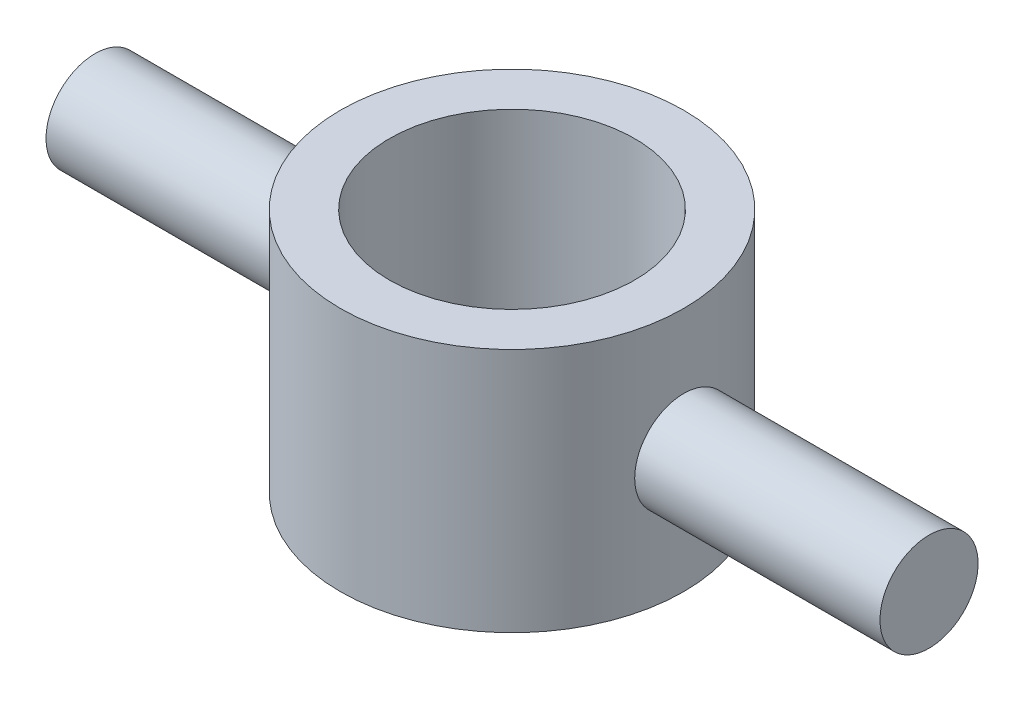
from build123d import *

# Parameters (mm, degrees)
SKETCH_2_R      = 7
SKETCH_2_R_2    = 5
EXTRUDE_1_DEPTH = 10
SKETCH_3_R      = 2
EXTRUDE_2_DEPTH = 10


with BuildPart() as part:
    # 草图2 → 凸台-拉伸1 (new body)
    with BuildSketch(Plane(origin=(0, 0, 0), x_dir=(1, 0, 0), z_dir=(0, 1, 0))):
        with Locations(Location((0, 0, 0), (0, 0, 270))):
            Circle(SKETCH_2_R)
        with Locations(Location((0, 0, 0), (0, 0, 270))):
            Circle(SKETCH_2_R_2, mode=Mode.SUBTRACT)
    extrude(amount=EXTRUDE_1_DEPTH)


with BuildPart() as body_2:
    # 草图3 → 凸台-拉伸2 (new body)
    with BuildSketch(Plane.ZY.offset(7)):
        with Locations((0, 5)):
            Circle(SKETCH_3_R)
    extrude(amount=EXTRUDE_2_DEPTH)


with BuildPart() as body_3:
    # 镜向3: mirrored copy
    add(body_2.part.mirror(Plane(origin=(0, 0, 0), x_dir=(0, 0, 1), z_dir=(1, 0, 0))))


solid = Compound([part.part, body_2.part, body_3.part])
